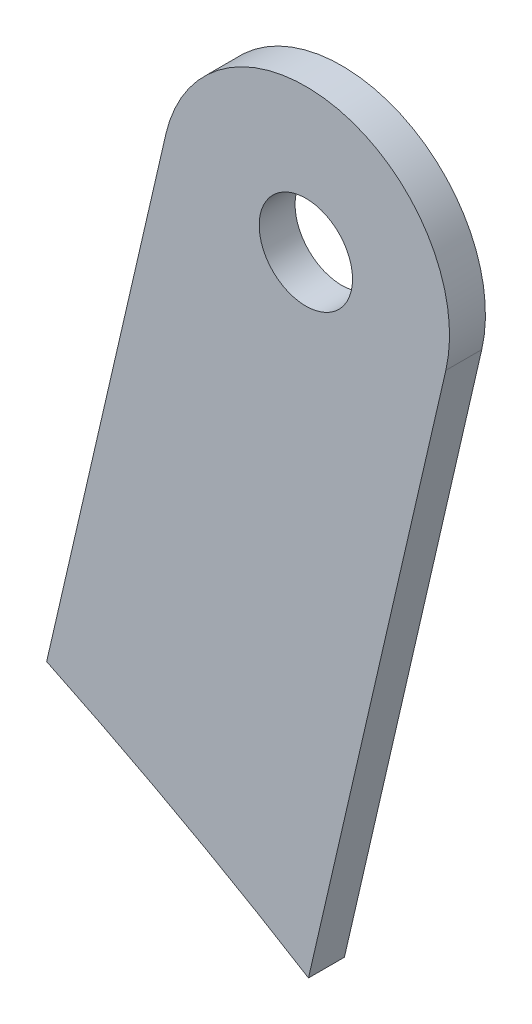
from build123d import *

# Parameters (mm, degrees)
SKETCH1_R           = 6.5
BOSS_EXTRUDE1_DEPTH = 2.5


with BuildPart() as part:
    # Sketch1 → Boss-Extrude1 (new, symmetric)
    with BuildSketch(Plane.XY):
        with BuildLine():
            Line((167.313008395, 349.517677982), (183.912598704, 421.418402931))
            ThreePointArc((183.912598704, 421.418402931), (207.899021087, 436.40678314), (222.887401296, 412.420360758))
            Line((222.887401296, 412.420360758), (203.766561676, 329.598905251))
            ThreePointArc((203.766561676, 329.598905251), (185.806892251, 340.047127311), (167.313008395, 349.517677982))
        make_face()
        with Locations((203.4, 416.919381844)):
            Circle(SKETCH1_R, mode=Mode.SUBTRACT)
    extrude(amount=BOSS_EXTRUDE1_DEPTH, both=True)


solid = part.part
